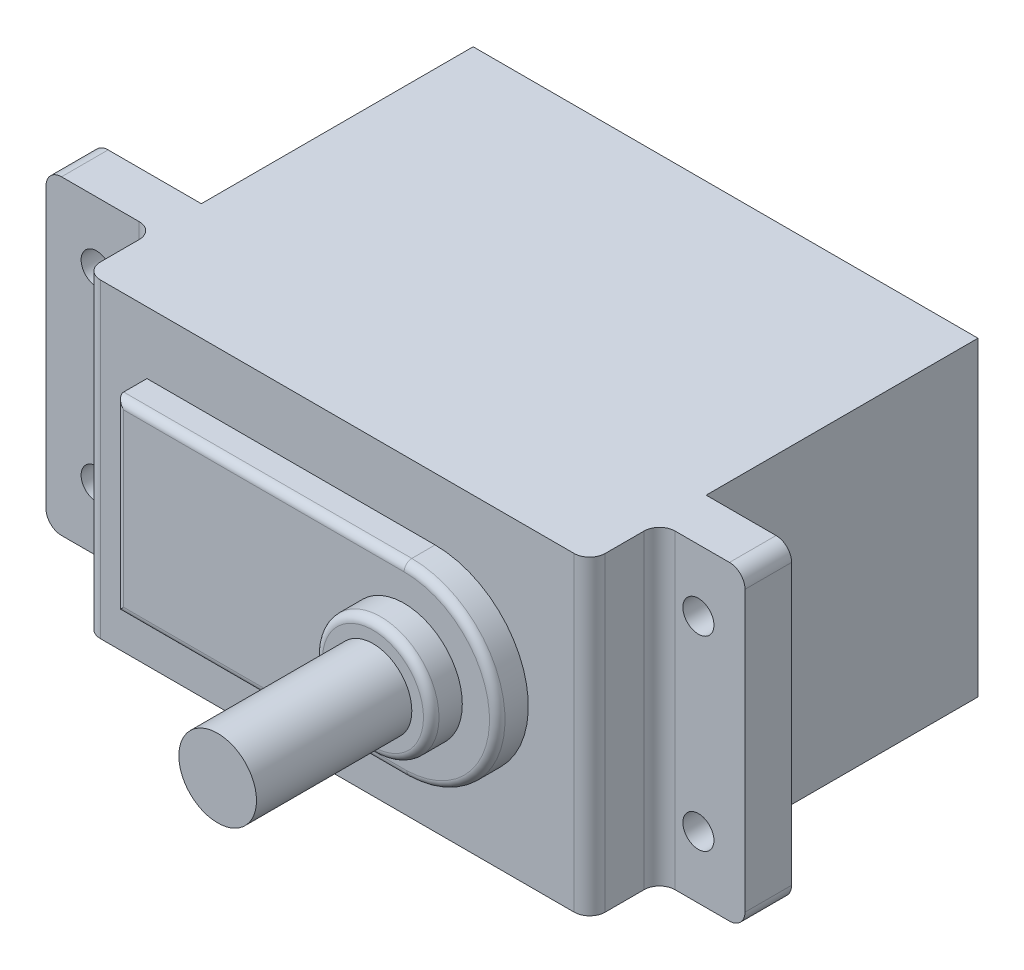
from build123d import *

# Parameters (mm, degrees)
SKETCH1_W           = 65
SKETCH1_H           = 40
BOSS_EXTRUDE1_DEPTH = 50
BOSS_EXTRUDE2_DEPTH = 4
SKETCH3_R           = 7.5
BOSS_EXTRUDE3_DEPTH = 4
SKETCH4_R           = 5
BOSS_EXTRUDE4_DEPTH = 20
FILLET1_R           = 1
SKETCH5_W           = 6
SKETCH5_H           = 40
BOSS_EXTRUDE5_DEPTH = 20
SKETCH6_W           = 6
SKETCH6_H           = 40
BOSS_EXTRUDE6_DEPTH = 20
SKETCH7_R           = 2
SKETCH7_W           = 9
SKETCH7_H           = 40
SKETCH7_W_2         = 6
CUT_EXTRUDE1_DEPTH  = 20
FILLET2_R           = 2
SCALE1_SCALE        = 0.5


with BuildPart() as part:
    # Sketch1 → Boss-Extrude1 (new body)
    with BuildSketch(Plane.XY):
        Rectangle(SKETCH1_W, SKETCH1_H)
    extrude(amount=BOSS_EXTRUDE1_DEPTH)

    # Sketch2 → Boss-Extrude2 (add)
    with BuildSketch(Plane.XY.offset(50)):
        with BuildLine():
            ThreePointArc((12.995819527, -11.993531793), (24.600254242, 0.197000611), (12.601871402, 12))
            Line((12.601871402, 12), (-24.5, 12))
            Line((-24.5, 12), (-24.5, -12.000098614))
            Line((-24.5, -12.000098614), (12.21212427, -11.993669046))
            Line((12.21212427, -11.993669046), (12.995819527, -11.993531793))
        make_face()
    extrude(amount=BOSS_EXTRUDE2_DEPTH)

    # Sketch3 → Boss-Extrude3 (add)
    with BuildSketch(Plane.XY.offset(54)):
        with Locations((12.601871402, 0)):
            Circle(SKETCH3_R)
    extrude(amount=BOSS_EXTRUDE3_DEPTH)

    # Sketch4 → Boss-Extrude4 (add)
    with BuildSketch(Plane.XY.offset(58)):
        with Locations((12.601871402, 0)):
            Circle(SKETCH4_R)
    extrude(amount=BOSS_EXTRUDE4_DEPTH)

    # Fillet1
    fillet1_edges = [part.edges().sort_by_distance(p)[0] for p in [
        (-5.752090236, -11.996815204, 54),
        (24.600254242, 0.197000611, 54),
        (-5.949064299, 12, 54),
        (-24.5, -4.9307e-05, 54),
        (5.101871402, 0, 58),
    ]]
    fillet(fillet1_edges, radius=FILLET1_R)

    # Sketch5 → Boss-Extrude5 (add)
    with BuildSketch(Plane(origin=(32.5, 0, 0), x_dir=(0, 0, -1), z_dir=(1, 0, 0))):
        with Locations((-38, 0)):
            Rectangle(SKETCH5_W, SKETCH5_H)
    extrude(amount=BOSS_EXTRUDE5_DEPTH)

    # Sketch6 → Boss-Extrude6 (add)
    with BuildSketch(Plane.ZY.offset(32.5)):
        with Locations((38, 0)):
            Rectangle(SKETCH6_W, SKETCH6_H)
    extrude(amount=BOSS_EXTRUDE6_DEPTH)

    # Sketch7 → Cut-Extrude1 (cut)
    with BuildSketch(Plane.XY.offset(41)):
        with Locations((-39.98, 12)):
            Circle(SKETCH7_R)
        with Locations((-39.98, -12)):
            Circle(SKETCH7_R)
        with Locations((37.5, 12)):
            Circle(SKETCH7_R)
        with Locations((37.5, -12)):
            Circle(SKETCH7_R)
        with Locations((48, 0)):
            Rectangle(SKETCH7_W, SKETCH7_H)
        with Locations((-49.5, 0)):
            Rectangle(SKETCH7_W_2, SKETCH7_H)
    extrude(amount=-CUT_EXTRUDE1_DEPTH, mode=Mode.SUBTRACT)

    # Fillet2
    fillet2_edges = [part.edges().sort_by_distance(p)[0] for p in [
        (32.5, 0, 50),
        (-46.5, 20, 38),
        (-46.5, -20, 38),
        (-32.5, 0, 50),
        (32.5, 0, 41),
        (-32.5, 0, 41),
        (43.5, -20, 38),
        (43.5, 20, 38),
    ]]
    fillet(fillet2_edges, radius=FILLET2_R)


with BuildPart() as part_1:
    # Scale1: scaled about (0, 0, 0)
    add(part.part.scale(SCALE1_SCALE))


solid = part_1.part
